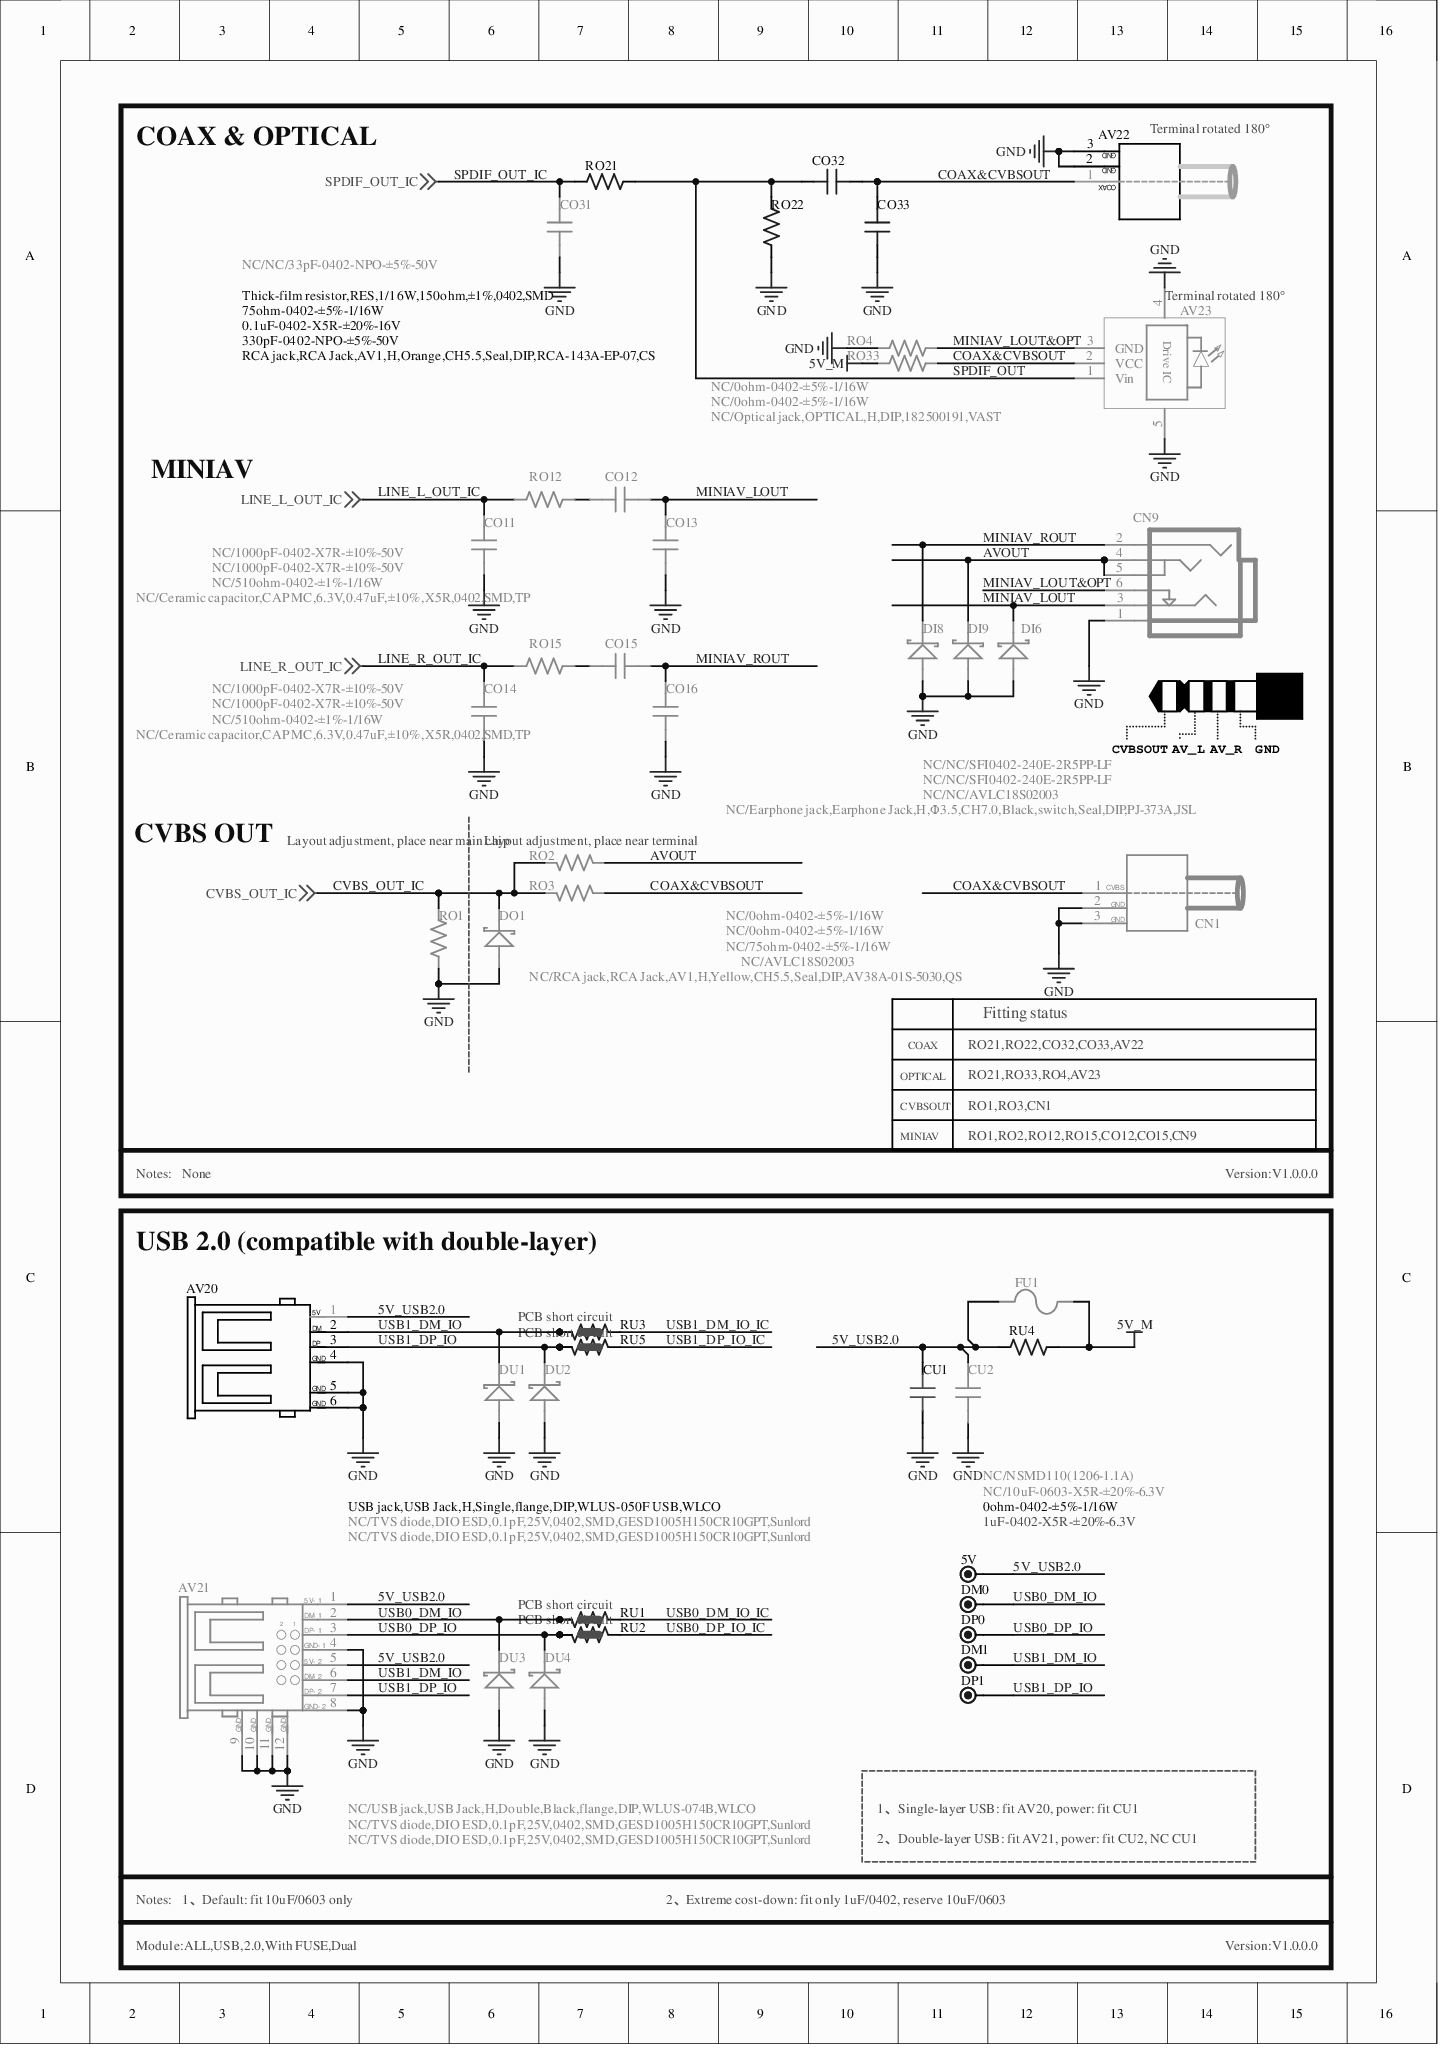
[diagram p0: MISC86372-13.SchDoc]
# Altium project MISC86372-32.PrjPCB (part 5 of 8)

## Sheet MISC86372-13.SchDoc
size 241 x 342 mm

### Parts
5V  DM0  [TP]  (value not drawn)
AV20  USB jack,USB Jack,H,Single,flange,DIP,WLUS-050F USB,WLCO  [USB1-HD-2]
AV21  NC/USB jack,USB Jack,H,Double,Black,flange,DIP,WLUS-074B,WLCO  [USB2-HD-1]
AV22  RCA jack,RCA Jack,AV1,H,Orange,CH5.5,Seal,DIP,RCA-143A-EP-07,CS  [AV1-H-4]
AV23  NC/Optical jack,OPTICAL,H,DIP,182500191,VAST  [OPTICAL-HD-3]
CN1  NC/RCA jack,RCA Jack,AV1,H,Yellow,CH5.5,Seal,DIP,AV38A-01S-5030,QS  [AV1-H-4]
CN9  NC/Earphone jack,Earphone Jack,H,Φ3.5,CH7.0,Black,switch,Seal,DIP,PJ-373A,JSL  [PHONE-HD-42]
CO11  NC/1000pF-0402-X7R-±10%-50V  [C0402]
CO12  NC/Ceramic capacitor,CAP MC,6.3V,0.47uF,±10%,X5R,0402,SMD,TP  [C0402]
CO13  NC/1000pF-0402-X7R-±10%-50V  [C0402]
CO14  NC/1000pF-0402-X7R-±10%-50V  [C0402]
CO15  NC/Ceramic capacitor,CAP MC,6.3V,0.47uF,±10%,X5R,0402,SMD,TP  [C0402]
CO16  NC/1000pF-0402-X7R-±10%-50V  [C0402]
CO31  NC/NC/33pF-0402-NPO-±5%-50V  [C0402]
CO32  0.1uF-0402-X5R-±20%-16V  [C0402]
CO33  330pF-0402-NPO-±5%-50V  [C0402]
CU1  1uF-0402-X5R-±20%-6.3V  [C0402]
CU2  NC/10uF-0603-X5R-±20%-6.3V  [C0603]
DI6  NC/NC/AVLC18S02003  [DIODE-S0402]
DI8  NC/NC/SFI0402-240E-2R5PP-LF  [DIODE-S0402]
DI9  NC/NC/SFI0402-240E-2R5PP-LF  [DIODE-S0402]
DM0  DM0  [TP]  (value not drawn)
DM1  DM0  [TP]  (value not drawn)
DO1  NC/AVLC18S02003  [DIODE-S0402]
DP0  DM0  [TP]  (value not drawn)
DP1  DM0  [TP]  (value not drawn)
DU1  NC/TVS diode,DIO ESD,0.1pF,25V,0402,SMD,GESD1005H150CR10GPT,Sunlord  [DIODE-S0402]
DU2  NC/TVS diode,DIO ESD,0.1pF,25V,0402,SMD,GESD1005H150CR10GPT,Sunlord  [DIODE-S0402]
DU3  NC/TVS diode,DIO ESD,0.1pF,25V,0402,SMD,GESD1005H150CR10GPT,Sunlord  [DIODE-S0402]
DU4  NC/TVS diode,DIO ESD,0.1pF,25V,0402,SMD,GESD1005H150CR10GPT,Sunlord  [DIODE-S0402]
FU1  NC/NSMD110(1206-1.1A)  [FUSE1.1A-S]
RO1  NC/75ohm-0402-±5%-1/16W  [R0402]
RO2  NC/0ohm-0402-±5%-1/16W  [R0402]
RO3  NC/0ohm-0402-±5%-1/16W  [R0402]
RO4  NC/0ohm-0402-±5%-1/16W  [R0402]
RO12  NC/510ohm-0402-±1%-1/16W  [R0402]
RO15  NC/510ohm-0402-±1%-1/16W  [R0402]
RO21  Thick-film resistor,RES,1/16W,150ohm,±1%,0402,SMD  [R0402]
RO22  75ohm-0402-±5%-1/16W  [R0402]
RO33  NC/0ohm-0402-±5%-1/16W  [R0402]
RU1  NC/0ohm-0402-PCB  [R0402SC]  (value not drawn)
RU2  NC/0ohm-0402-PCB  [R0402SC]  (value not drawn)
RU3  NC/0ohm-0402-PCB  [R0402SC]  (value not drawn)
RU4  0ohm-0402-±5%-1/16W  [R0402]
RU5  NC/0ohm-0402-PCB  [R0402SC]  (value not drawn)

### Blocks framed on the sheet
USB 2.0 (compatible with double-layer): 5V AV20 AV21 CU1 CU2 DM0 DM1 DP0 DP1 DU1-DU4 FU1 RU1-RU5

### Nets
5V_M: FU1.2 RO33.1 RU4.2
GND: AV20.4 AV20.5 AV20.6 AV21.4 AV21.8 AV21.9 AV21.10 AV21.11 AV21.12 AV22.2(GND) AV22.3(GND) AV23.4(GND) AV23.5(GND) CN1.2(GND) CN1.3(GND) CN9.1 CO11.1 CO13.1 CO14.1 CO16.1 CO31.1 CO33.1 CU1.2 CU2.2 DI6.A DI8.A DI9.A DO1.A DU1.A DU2.A DU3.A DU4.A RO1.1 RO4.1 RO22.1
5V_USB2.0: 5V.1 AV20.1 AV21.1 AV21.5 CU1.1 CU2.1 FU1.1 RU4.1
AVOUT: CN9.4 CN9.5 DI9.K RO2.1
COAX&CVBSOUT: AV22.1(CVBS) AV23.2(VCC) CN1.1(CVBS) CO32.1 CO33.2 RO3.1 RO33.2
CVBS_OUT_IC: DO1.K RO1.2 RO2.2 RO3.2 ; off-sheet CVBS_OUT_IC
LINE_L_OUT_IC: CO11.2 RO12.2 ; off-sheet LINE_L_OUT_IC
LINE_R_OUT_IC: CO14.2 RO15.2 ; off-sheet LINE_R_OUT_IC
MINIAV_LOUT: CN9.3 CO12.1 CO13.2 DI6.K
MINIAV_LOUT&OPT: AV23.3(GND) CN9.6 RO4.2
MINIAV_ROUT: CN9.2 CO15.1 CO16.2 DI8.K
SPDIF_OUT: AV23.1(Vin) CO32.2 RO21.2 RO22.2
SPDIF_OUT_IC: CO31.2 RO21.1 ; off-sheet SPDIF_OUT_IC
USB0_DM_IO: AV21.2 DM0.1 DU3.K RU1.2 RU1.3
USB0_DM_IO_IC: RU1.1
USB0_DP_IO: AV21.3 DP0.1 DU4.K RU2.2 RU2.3
USB0_DP_IO_IC: RU2.1
USB1_DM_IO: AV20.2 AV21.6 DM1.1 DU1.K RU3.2 RU3.3
USB1_DM_IO_IC: RU3.1
USB1_DP_IO: AV20.3 AV21.7 DP1.1 DU2.K RU5.2 RU5.3
USB1_DP_IO_IC: RU5.1
NetCO12_2: CO12.2 RO12.1
NetCO15_2: CO15.2 RO15.1

### Notes on the sheet
- COAX & OPTICAL
- (near AV22) Terminal rotated 180°
- (near AV23) Terminal rotated 180°
- MINIAV
- CVBSOUT
- AV_L
- AV_R
- GND
- CVBS OUT
- (near RO2) Layout adjustment, place near main chip
- (near RO2) Layout adjustment, place near terminal
- Fitting status
- OPTICAL
- COAX
- RO21,RO22,CO32,CO33,AV22
- RO21,RO33,RO4,AV23
- RO1,RO3,CN1
- RO1,RO2,RO12,RO15,CO12,CO15,CN9
- Notes:
- None
- Version:V1.0.0.0
- 1、 Single-layer USB: fit AV20, power: fit CU1
- 2、 Double-layer USB: fit AV21, power: fit CU2, NC CU1
- 1、 Default: fit 10uF/0603 only
- 2、 Extreme cost-down: fit only 1uF/0402, reserve 10uF/0603
- Module:ALL,USB,2.0,With FUSE,Dual

### Library data of the parts
5V DM0 DM1 DP0 DP1 = TEST
AV20 = XXX.XXX.0002687: USB jack,USB Jack,H,Single,flange,DIP,103411271,VAST-DLMI
AV21 = XXX.XXX.0001070-DLMI: USB jack,USB Jack,H,Double,Black,flange,DIP,WLUS-074B,WLCO-DLMI; Revision: *
AV22 = RCA端子,RCA Jack,AV1,H,Orange,CH5.5,Seal,DIP,AV38A-01S-5020,QS-DLMI
AV23 = 光纤端子,OPTICAL,H,DIP,GQ-03-08C1,QS-DLMI: CN-DLMI-optical fibre
CN1 = RCA端子,RCA Jack,AV1,H,Yellow,CH5.5,Seal,DIP,AV38A-01S-5030,QS-DLMI
CN9 = XXX.XXX.0002138: Earphone jack,Earphone Jack,H,Φ3.5,CH7.0,Black,switch,Seal,DIP,PJ7724-F05L3BY-D,YUQIU-DLMI
CO11 CO13 CO14 CO16 = 1000pF-0402-X7R-±10%-50V-D
CO12 CO15 = 004.003.0000361-D: Ceramic capacitor,CAP MC,6.3V,0.47uF,±10%,X5R,0402,SMD,TP-D
CO31 = 33pF-0402-NPO-±5%-50V-D
CO32 = 004.003.0000403-D: Ceramic capacitor,CAP MC,16V,0.1uF,±20%,X5R,0402,SMD,TP-D
CO33 = 330pF-0402-NPO-±5%-50V-D
CU1 = 1uF-0402-X5R-±20%-6.3V-D
CU2 = 10uF-0603-X5R-±20%-6.3V-D
DI6 DO1 = AVLC18S02003-D
DI8 DI9 = SFI0402-240E-2R5PP-LF-D
DU1-DU4 = 004.005.0000203-D: TVS diode,DIO ESD,0.2pF,25V,0402,SMD,AIES12U020R2,AMOTECH-D
FU1 = 004.026.0000039-D: Self-recovering fuse,FUSE PTC,1.1A,6V,1206,SMD,TP,TLC-D
RO1 = 75ohm-0402-±5%-1/16W-D
RO2 RO3 RU4 = 004.002.0000558-D: Thick-film resistor,RES,1/16W,0ohm,±5%,0402,SMD-D
RO4 RO33 = 0ohm-0402-±5%-1/16W-D
RO12 RO15 = 510ohm-0402-±5%-1/16W-D
RO21 = 004.002.0000609-D: Thick-film resistor,RES,1/16W,180ohm,±5%,0402,SMD-D
RO22 = 004.002.0000568-D: Thick-film resistor,RES,1/16W,100ohm,±5%,0402,SMD-D
RU1-RU3 RU5 = 0ohm-0402-PCB-D

## Sheet MISC86372-14.SchDoc
size 393 x 368 mm
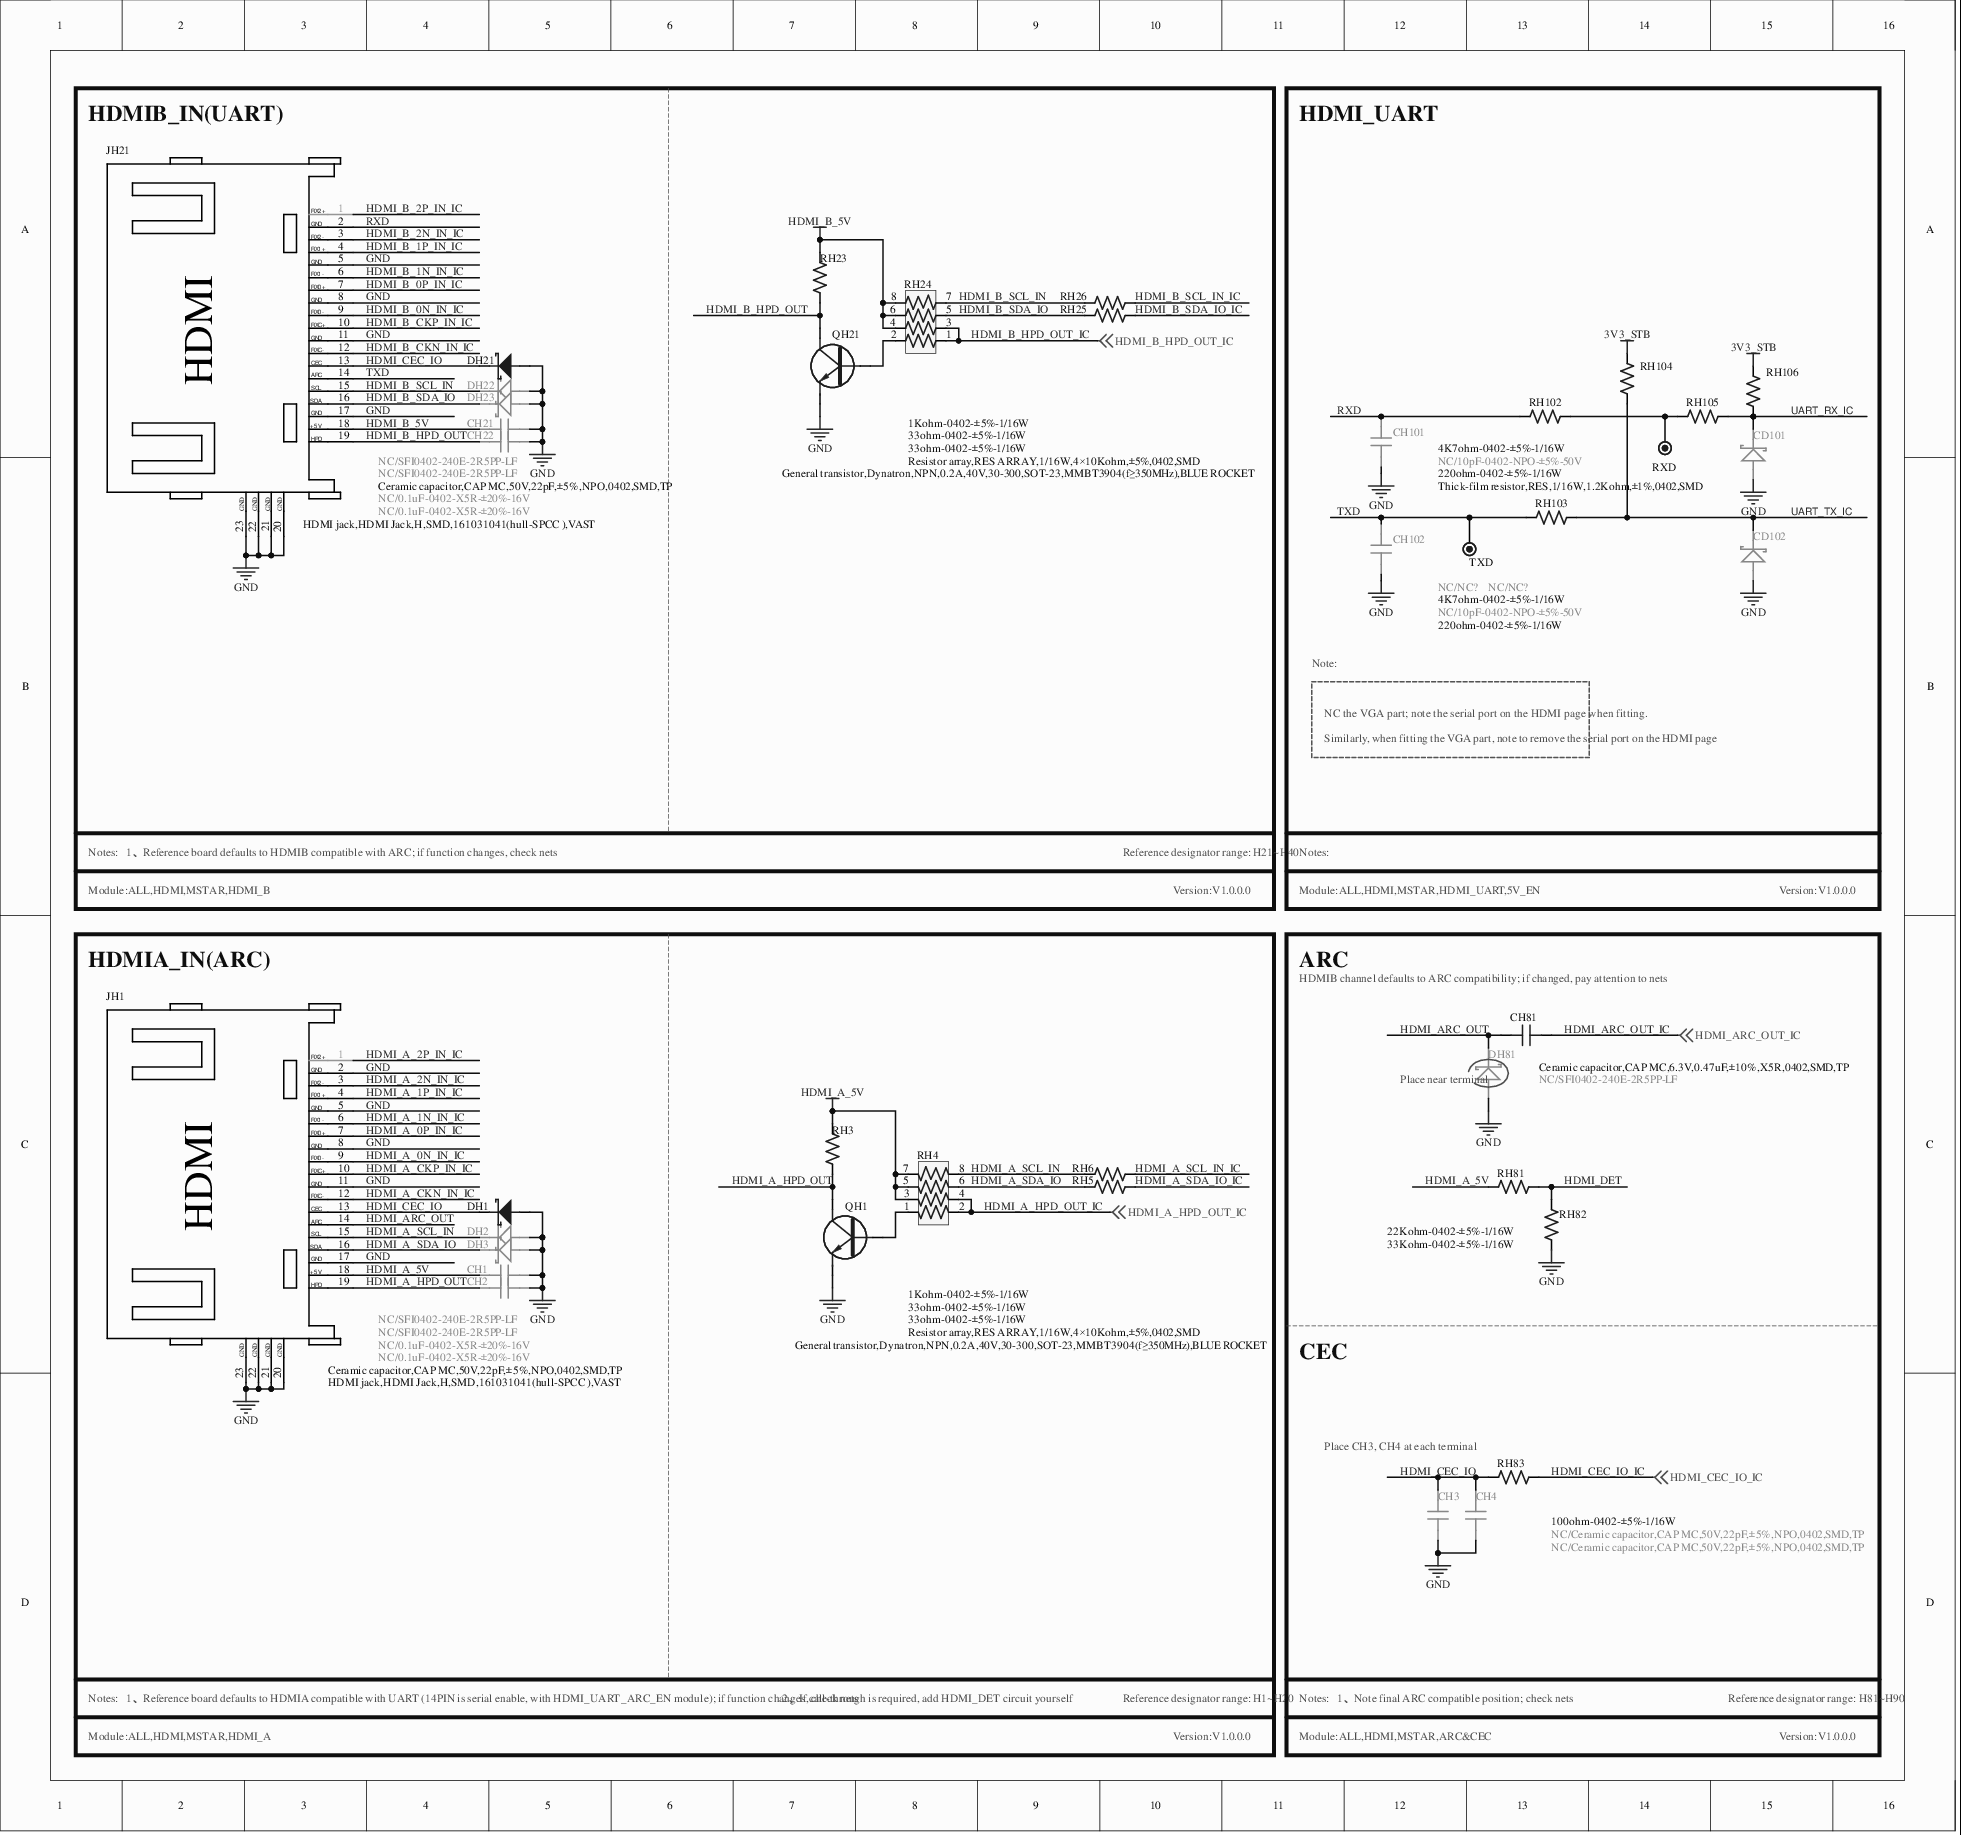
[diagram p1: MISC86372-14.SchDoc]

### Parts
CD101  NC/NC?  [DIODE-S0402]
CD102  NC/NC?  [DIODE-S0402]
CH1  NC/0.1uF-0402-X5R-±20%-16V  [C0402]
CH2  NC/0.1uF-0402-X5R-±20%-16V  [C0402]
CH3  NC/Ceramic capacitor,CAP MC,50V,22pF,±5%,NPO,0402,SMD,TP  [C0402]
CH4  NC/Ceramic capacitor,CAP MC,50V,22pF,±5%,NPO,0402,SMD,TP  [C0402]
CH21  NC/0.1uF-0402-X5R-±20%-16V  [C0402]
CH22  NC/0.1uF-0402-X5R-±20%-16V  [C0402]
CH81  Ceramic capacitor,CAP MC,6.3V,0.47uF,±10%,X5R,0402,SMD,TP  [C0402]
CH101  NC/10pF-0402-NPO-±5%-50V  [C0402]
CH102  NC/10pF-0402-NPO-±5%-50V  [C0402]
DH1  Ceramic capacitor,CAP MC,50V,22pF,±5%,NPO,0402,SMD,TP  [DIODE-S0402]
DH2  NC/SFI0402-240E-2R5PP-LF  [DIODE-S0402]
DH3  NC/SFI0402-240E-2R5PP-LF  [DIODE-S0402]
DH21  Ceramic capacitor,CAP MC,50V,22pF,±5%,NPO,0402,SMD,TP  [DIODE-S0402]
DH22  NC/SFI0402-240E-2R5PP-LF  [DIODE-S0402]
DH23  NC/SFI0402-240E-2R5PP-LF  [DIODE-S0402]
DH81  NC/SFI0402-240E-2R5PP-LF  [DIODE-S0402]
JH1  HDMI jack,HDMI Jack,H,SMD,161031041(hull-SPCC ),VAST  [HDMI-HS-1]
JH21  HDMI jack,HDMI Jack,H,SMD,161031041(hull-SPCC ),VAST  [HDMI-HS-1]
QH1  General transistor,Dynatron,NPN,0.2A,40V,30-300,SOT-23,MMBT3904(f≥350MHz),BLUE ROCKET  [SOT-23]
QH21  General transistor,Dynatron,NPN,0.2A,40V,30-300,SOT-23,MMBT3904(f≥350MHz),BLUE ROCKET  [SOT-23]
RH3  1Kohm-0402-±5%-1/16W  [R0402]
RH4  Resistor array,RES ARRAY,1/16W,4×10Kohm,±5%,0402,SMD  [RA0402]
RH5  33ohm-0402-±5%-1/16W  [R0402]
RH6  33ohm-0402-±5%-1/16W  [R0402]
RH23  1Kohm-0402-±5%-1/16W  [R0402]
RH24  Resistor array,RES ARRAY,1/16W,4×10Kohm,±5%,0402,SMD  [RA0402]
RH25  33ohm-0402-±5%-1/16W  [R0402]
RH26  33ohm-0402-±5%-1/16W  [R0402]
RH81  22Kohm-0402-±5%-1/16W  [R0402]
RH82  33Kohm-0402-±5%-1/16W  [R0402]
RH83  100ohm-0402-±5%-1/16W  [R0402]
RH102  Thick-film resistor,RES,1/16W,1.2Kohm,±1%,0402,SMD  [R0402]
RH103  220ohm-0402-±5%-1/16W  [R0402]
RH104  4K7ohm-0402-±5%-1/16W  [R0402]
RH105  220ohm-0402-±5%-1/16W  [R0402]
RH106  4K7ohm-0402-±5%-1/16W  [R0402]
RXD  (no value)  [TP]
TXD  (no value)  [TP]

### Blocks framed on the sheet
HDMIB_IN(UART): CH21 CH22 DH21-DH23 JH21 QH21 RH23-RH26
HDMI_UART: CD101 CD102 CH101 CH102 RH102-RH106 RXD TXD
HDMIA_IN(ARC): CH1 CH2 DH1-DH3 JH1 QH1 RH3-RH6

### Nets
3V3_STB: RH104.2 RH106.2
GND: CD101.A CD102.A CH1.2 CH2.2 CH3.1 CH4.1 CH21.2 CH22.2 CH101.1 CH102.1 DH1.A DH2.A DH3.A DH21.A DH22.A DH23.A DH81.A JH1.2 JH1.5 JH1.8 JH1.11 JH1.17 JH1.20 JH1.21 JH1.22 JH1.23 JH21.5 JH21.8 JH21.11 JH21.17 JH21.20 JH21.21 JH21.22 JH21.23 QH1.E QH21.E RH82.2
HDMI_A_5V: CH1.1 JH1.18 RH3.2 RH4.3 RH4.5 RH4.7 RH81.2
HDMI_B_5V: CH21.1 JH21.18 RH23.2 RH24.4 RH24.6 RH24.8
HDMI_A_0N_IN_IC: JH1.9
HDMI_A_0P_IN_IC: JH1.7
HDMI_A_1N_IN_IC: JH1.6
HDMI_A_1P_IN_IC: JH1.4
HDMI_A_2N_IN_IC: JH1.3
HDMI_A_2P_IN_IC: JH1.1
HDMI_A_CKN_IN_IC: JH1.12
HDMI_A_CKP_IN_IC: JH1.10
HDMI_A_HPD_OUT: CH2.1 JH1.19 QH1.C RH3.1
HDMI_A_HPD_OUT_IC: RH4.2 RH4.4 ; off-sheet HDMI_A_HPD_OUT_IC
HDMI_A_SCL_IN: DH2.K JH1.15 RH4.8 RH6.1
HDMI_A_SCL_IN_IC: RH6.2
HDMI_A_SDA_IO: DH3.K JH1.16 RH4.6 RH5.1
HDMI_A_SDA_IO_IC: RH5.2
HDMI_ARC_OUT: CH81.1 DH81.K JH1.14
HDMI_ARC_OUT_IC: CH81.2 ; off-sheet HDMI_ARC_OUT_IC
HDMI_B_0N_IN_IC: JH21.9
HDMI_B_0P_IN_IC: JH21.7
HDMI_B_1N_IN_IC: JH21.6
HDMI_B_1P_IN_IC: JH21.4
HDMI_B_2N_IN_IC: JH21.3
HDMI_B_2P_IN_IC: JH21.1
HDMI_B_CKN_IN_IC: JH21.12
HDMI_B_CKP_IN_IC: JH21.10
HDMI_B_HPD_OUT: CH22.1 JH21.19 QH21.C RH23.1
HDMI_B_HPD_OUT_IC: RH24.1 RH24.3 ; off-sheet HDMI_B_HPD_OUT_IC
HDMI_B_SCL_IN: DH22.K JH21.15 RH24.7 RH26.1
HDMI_B_SCL_IN_IC: RH26.2
HDMI_B_SDA_IO: DH23.K JH21.16 RH24.5 RH25.1
HDMI_B_SDA_IO_IC: RH25.2
HDMI_CEC_IO: CH3.2 CH4.2 DH1.K DH21.K JH1.13 JH21.13 RH83.2
HDMI_CEC_IO_IC: RH83.1 ; off-sheet HDMI_CEC_IO_IC
HDMI_DET: RH81.1 RH82.1
RXD: CH101.2 JH21.2 RH102.1
TXD: CH102.2 JH21.14 RH103.1 TXD.1
UART_RX_IC: CD101.K RH105.2 RH106.1
UART_TX_IC: CD102.K RH103.2 RH104.1
NetQH1_B: QH1.B RH4.1
NetQH21_B: QH21.B RH24.2
NetRH102_2: RH102.2 RH105.1 RXD.1

### Notes on the sheet
- Note:
- NC the VGA part; note the serial port on the HDMI page when fitting.
- Similarly, when fitting the VGA part, note to remove the serial port on the HDMI page
- Module:ALL,HDMI,MSTAR,HDMI_B
- Notes:
- 1、 Reference board defaults to HDMIB compatible with ARC; if function changes, check nets
- Reference designator range: H21~H40
- Version:V1.0.0.0
- Module:ALL,HDMI,MSTAR,HDMI_UART,5V_EN
- ARC
- HDMIB channel defaults to ARC compatibility; if changed, pay attention to nets
- (near DH81) Place near terminal
- CEC
- (near RH83) Place CH3, CH4 at each terminal
- 1、 Reference board defaults to HDMIA compatible with UART (14PIN is serial enable, with HDMI_UART_ARC_EN module); if function changes, check nets
- 2、 If call-through is required, add HDMI_DET circuit yourself
- Reference designator range: H1~H20
- 1、 Note final ARC compatible position; check nets
- Reference designator range: H81~H90
- Module:ALL,HDMI,MSTAR,HDMI_A
- Module:ALL,HDMI,MSTAR,ARC&CEC

### Library data of the parts
CD101 CD102 = AVLC18S02003-D
CH1 CH2 CH21 CH22 = 0.1uF-0402-X5R-±20%-16V-D
CH3 CH4 = 004.003.0000530-D: Ceramic capacitor,CAP MC,50V,22pF,±5%,NPO,0402,SMD,TP-D
CH81 = 1uF-0402-X5R-±20%-6.3V-D
CH101 CH102 = 220pF-0402-X7R-±10%-50V-D
DH1-DH3 DH21-DH23 DH81 = 004.005.0000315-D: TVS diode,DIO ESD,2.5pF,200V,0402,SMD,SFI0402-240E-2R5PP-LF,SFI-D
JH1 JH21 = XXX.XXX.0001122-D: HDMI jack,HDMI Jack,H,SMD,161031041(hull-SPCC ),VAST-D
QH1 QH21 = 004.006.0000007-D: General transistor,Dynatron,NPN,0.2A,40V,60-300,SOT-23,KMBT3904,KEXIN-D
RH3 RH23 = 1Kohm-0402-±5%-1/16W-D
RH4 RH24 = 4*100ohm-0402-±5%-1/16W-D
RH5 RH6 RH25 RH26 = 33ohm-0402-±5%-1/16W-D
RH81 = 22Kohm-0402-±5%-1/16W-D
RH82 = 33Kohm-0402-±5%-1/16W-D
RH83 = 004.002.0000568-D: as RO22 on sheet MISC86372-13
RH102-RH106 = 68ohm-0402-±5%-1/16W-D
RXD TXD = TEST

## Sheet MISC86372-15.SchDoc
size 294 x 304 mm
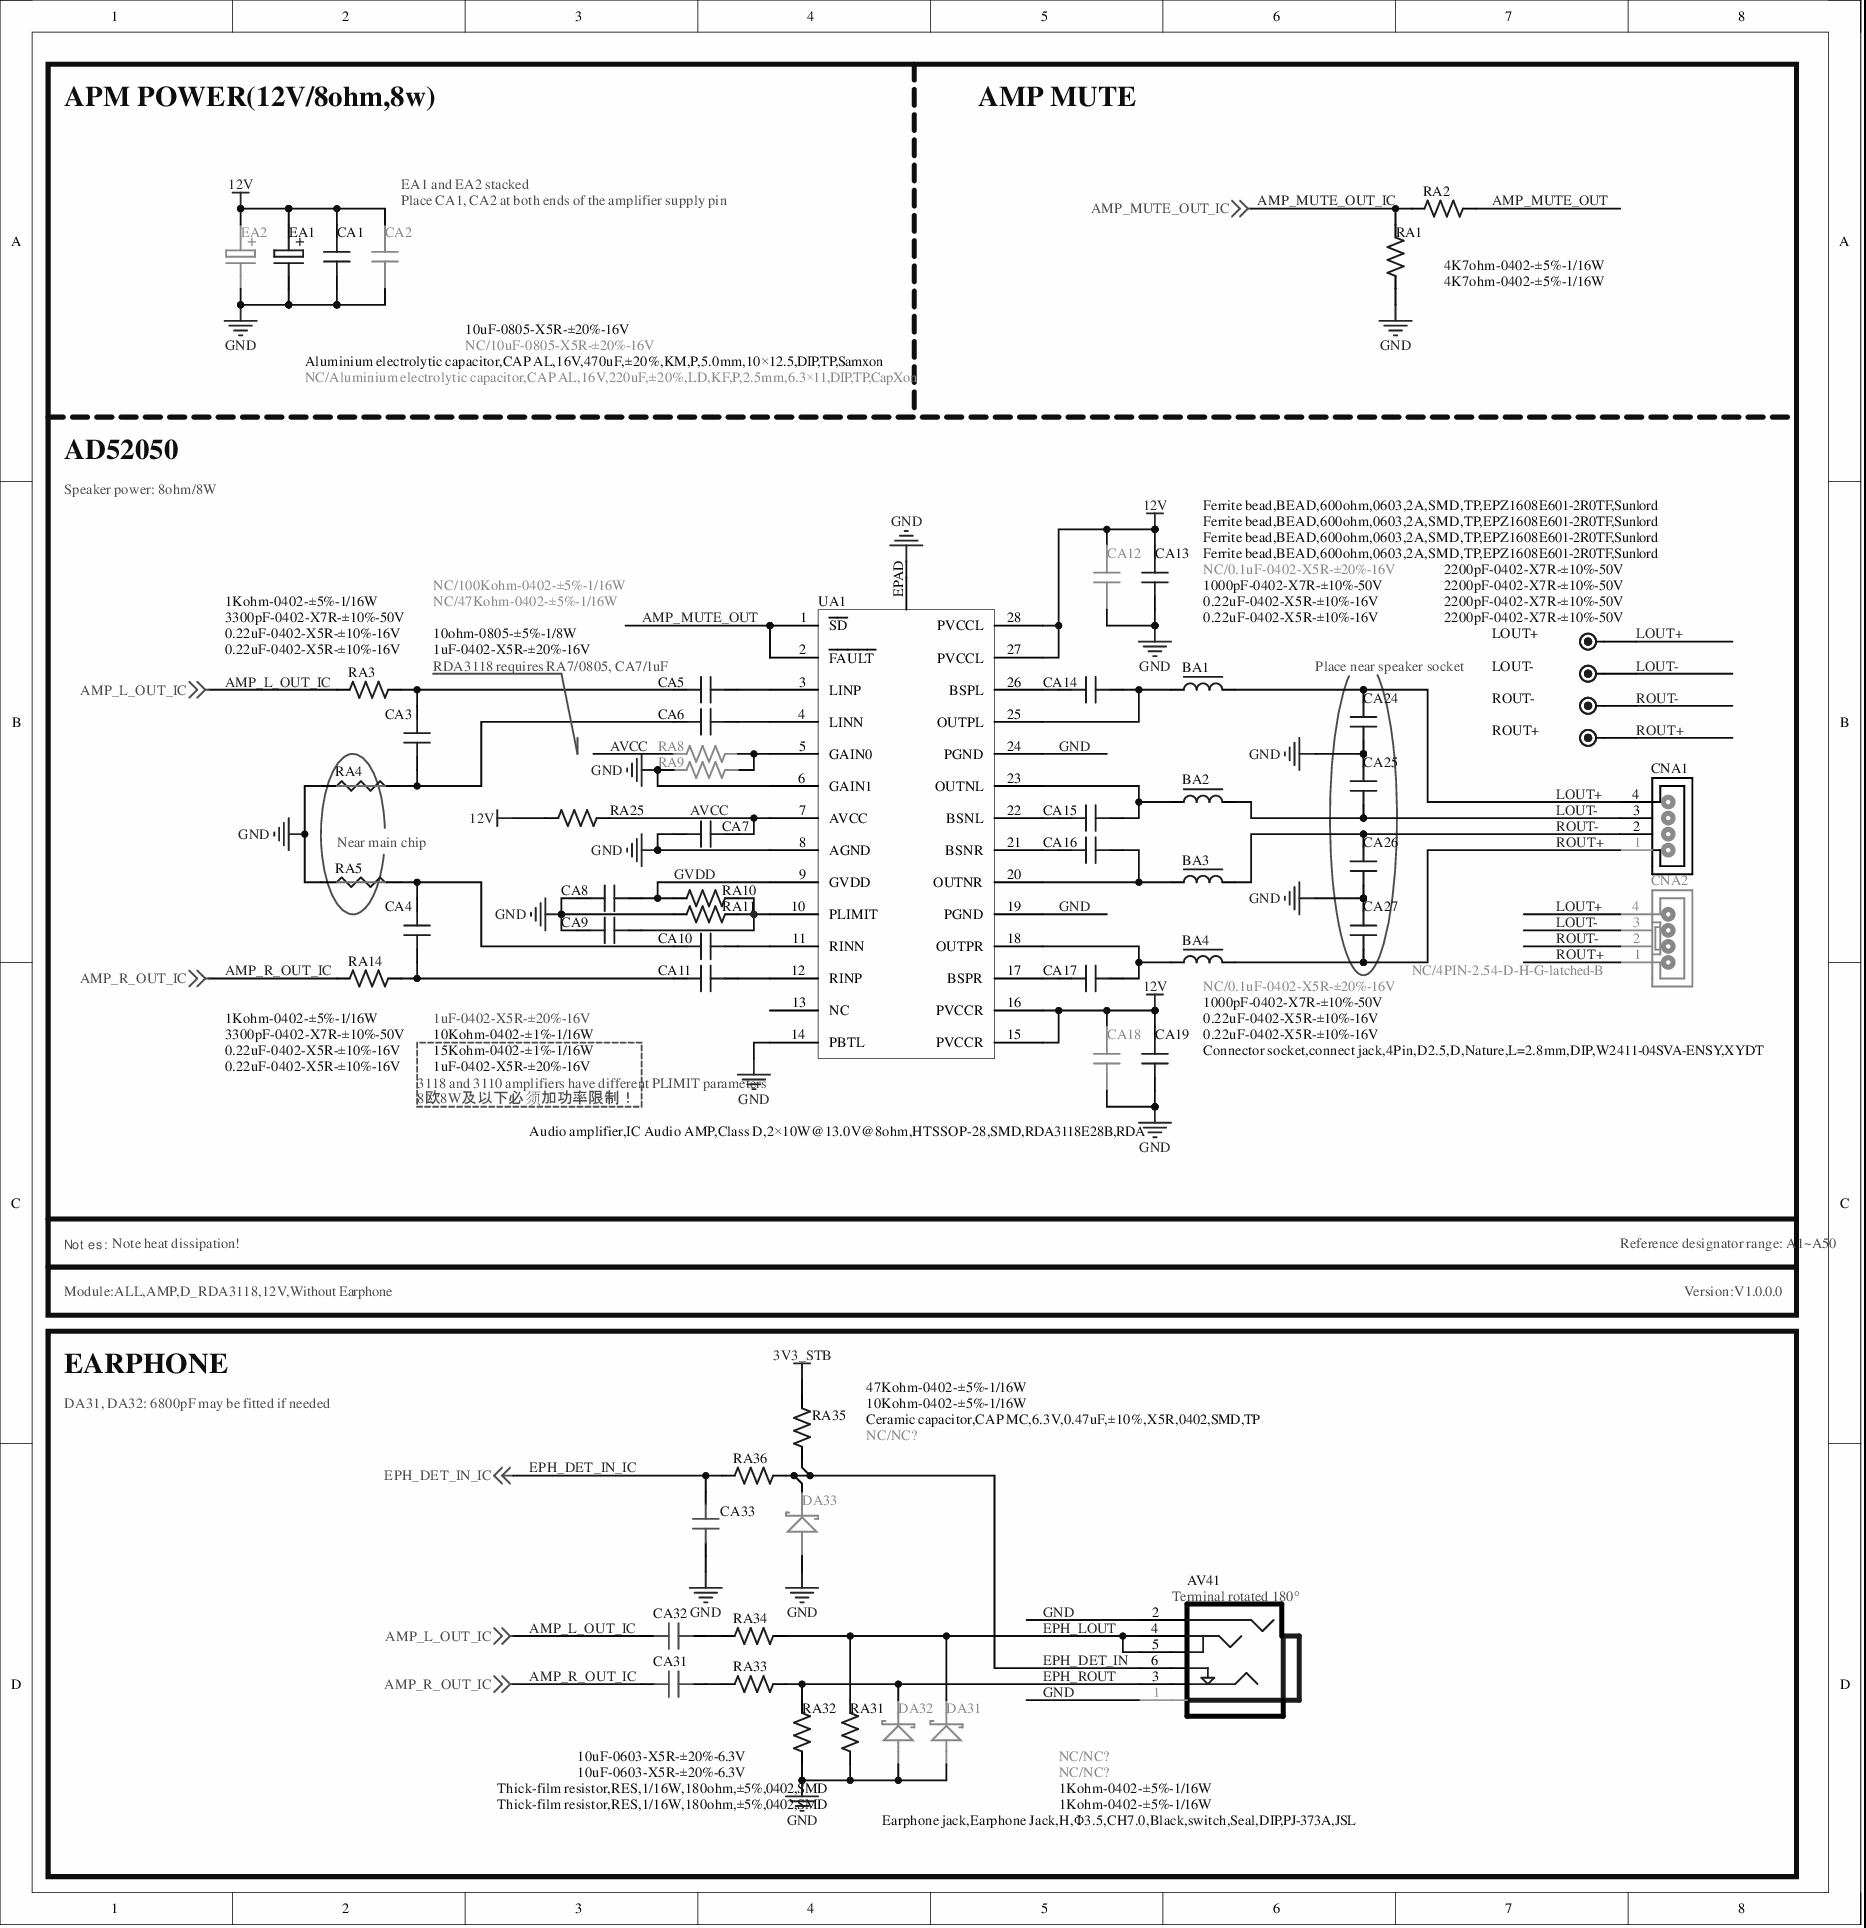
[diagram p2: MISC86372-15.SchDoc]

### Parts
AV41  Earphone jack,Earphone Jack,H,Φ3.5,CH7.0,Black,switch,Seal,DIP,PJ-373A,JSL  [PHONE-HD-42]
BA1  Ferrite bead,BEAD,600ohm,0603,2A,SMD,TP,EPZ1608E601-2R0TF,Sunlord  [L0603]
BA2  Ferrite bead,BEAD,600ohm,0603,2A,SMD,TP,EPZ1608E601-2R0TF,Sunlord  [L0603]
BA3  Ferrite bead,BEAD,600ohm,0603,2A,SMD,TP,EPZ1608E601-2R0TF,Sunlord  [L0603]
BA4  Ferrite bead,BEAD,600ohm,0603,2A,SMD,TP,EPZ1608E601-2R0TF,Sunlord  [L0603]
CA1  10uF-0805-X5R-±20%-16V  [C0805]
CA2  NC/10uF-0805-X5R-±20%-16V  [C0805]
CA3  3300pF-0402-X7R-±10%-50V  [C0402]
CA4  3300pF-0402-X7R-±10%-50V  [C0402]
CA5  0.22uF-0402-X5R-±10%-16V  [C0402]
CA6  0.22uF-0402-X5R-±10%-16V  [C0402]
CA7  1uF-0402-X5R-±20%-16V  [C0402]
CA8  1uF-0402-X5R-±20%-16V  [C0402]
CA9  1uF-0402-X5R-±20%-16V  [C0402]
CA10  0.22uF-0402-X5R-±10%-16V  [C0402]
CA11  0.22uF-0402-X5R-±10%-16V  [C0402]
CA12  NC/0.1uF-0402-X5R-±20%-16V  [C0402]
CA13  1000pF-0402-X7R-±10%-50V  [C0402]
CA14  0.22uF-0402-X5R-±10%-16V  [C0402]
CA15  0.22uF-0402-X5R-±10%-16V  [C0402]
CA16  0.22uF-0402-X5R-±10%-16V  [C0402]
CA17  0.22uF-0402-X5R-±10%-16V  [C0402]
CA18  NC/0.1uF-0402-X5R-±20%-16V  [C0402]
CA19  1000pF-0402-X7R-±10%-50V  [C0402]
CA24  2200pF-0402-X7R-±10%-50V  [C0402]
CA25  2200pF-0402-X7R-±10%-50V  [C0402]
CA26  2200pF-0402-X7R-±10%-50V  [C0402]
CA27  2200pF-0402-X7R-±10%-50V  [C0402]
CA31  10uF-0603-X5R-±20%-6.3V  [C0603]
CA32  10uF-0603-X5R-±20%-6.3V  [C0603]
CA33  Ceramic capacitor,CAP MC,6.3V,0.47uF,±10%,X5R,0402,SMD,TP  [C0402]
CNA1  Connector socket,connect jack,4Pin,D2.5,D,Nature,L=2.8mm,DIP,W2411-04SVA-ENSY,XYDT  [SIP4/2.54D-1]
CNA2  NC/4PIN-2.54-D-H-G-latched-B  [SIP4/2.5D-2]
DA31  NC/NC?  [DIODE-S0402]
DA32  NC/NC?  [DIODE-S0402]
DA33  NC/NC?  [DIODE-S0402]
EA1  Aluminium electrolytic capacitor,CAP AL,16V,470uF,±20%,KM,P,5.0mm,10×12.5,DIP,TP,Samxon  [EC(10*12)-V-5]
EA2  NC/Aluminium electrolytic capacitor,CAP AL,16V,220uF,±20%,LD,KF,P,2.5mm,6.3×11,DIP,TP,CapXon  [EC(6.3*11)-V-2.5]
LOUT+  DM0  [TP]  (value not drawn)
LOUT-  DM0  [TP]  (value not drawn)
RA1  4K7ohm-0402-±5%-1/16W  [R0402]
RA2  4K7ohm-0402-±5%-1/16W  [R0402]
RA3  1Kohm-0402-±5%-1/16W  [R0402]
RA4  NC/?  [GND]  (value not drawn)
RA5  NC/?  [GND]  (value not drawn)
RA8  NC/100Kohm-0402-±5%-1/16W  [R0402]
RA9  NC/47Kohm-0402-±5%-1/16W  [R0402]
RA10  10Kohm-0402-±1%-1/16W  [R0402]
RA11  15Kohm-0402-±1%-1/16W  [R0402]
RA14  1Kohm-0402-±5%-1/16W  [R0402]
RA25  10ohm-0805-±5%-1/8W  [R0805]
RA31  1Kohm-0402-±5%-1/16W  [R0402]
RA32  1Kohm-0402-±5%-1/16W  [R0402]
RA33  Thick-film resistor,RES,1/16W,180ohm,±5%,0402,SMD  [R0402]
RA34  Thick-film resistor,RES,1/16W,180ohm,±5%,0402,SMD  [R0402]
RA35  47Kohm-0402-±5%-1/16W  [R0402]
RA36  10Kohm-0402-±5%-1/16W  [R0402]
ROUT+  DM0  [TP]  (value not drawn)
ROUT-  DM0  [TP]  (value not drawn)
UA1  Audio amplifier,IC Audio AMP,Class D,2×10W@13.0V@8ohm,HTSSOP-28,SMD,RDA3118E28B,RDA  [SSOP28/0.65-5]

### Blocks framed on the sheet
EARPHONE: AV41 CA31-CA33 DA31-DA33 RA31-RA36

### Nets
3V3_STB: RA35.2
12V: CA1.2 CA2.2 CA12.2 CA13.2 CA18.2 CA19.2 EA1.1 EA2.1 RA25.1 UA1.15(PVCCR) UA1.16(PVCCR) UA1.27(PVCCL) UA1.28(PVCCL)
GND: AV41.1 AV41.2 CA1.1 CA2.1 CA7.1 CA8.1 CA9.1 CA12.1 CA13.1 CA18.1 CA19.1 CA24.1 CA25.2 CA26.1 CA27.2 CA33.1 DA31.A DA32.A DA33.A EA1.2 EA2.2 RA1.2 RA4.JP_2K RA5.JP_2K RA9.1 RA11.1 RA31.1 RA32.1 UA1.6(GAIN1) UA1.8(AGND) UA1.14(PBTL) UA1.19(PGND) UA1.24(PGND) UA1.EPAD
AMP_L_OUT_IC: CA32.2 RA3.1 ; off-sheet AMP_L_OUT_IC
AMP_MUTE_OUT: RA2.1 UA1.1(~{SD}) UA1.2(~{FAULT})
AMP_MUTE_OUT_IC: RA1.1 RA2.2 ; off-sheet AMP_MUTE_OUT_IC
AMP_R_OUT_IC: CA31.2 RA14.1 ; off-sheet AMP_R_OUT_IC
AVCC: CA7.2 RA8.1 RA25.2 UA1.7(AVCC)
EPH_DET_IN: AV41.6 DA33.K RA35.1 RA36.2
EPH_DET_IN_IC: CA33.2 RA36.1 ; off-sheet EPH_DET_IN_IC
EPH_LOUT: AV41.4 AV41.5 DA31.K RA31.2 RA34.2
EPH_ROUT: AV41.3 DA32.K RA32.2 RA33.2
GVDD: CA8.2 RA10.1 UA1.9(GVDD)
LOUT+: BA1.2 CA24.2 CNA1.4 CNA2.4 LOUT+.1
LOUT-: BA2.2 CA25.1 CNA1.3 CNA2.3 LOUT-.1
ROUT+: BA4.2 CA27.1 CNA1.1 CNA2.1 ROUT+.1
ROUT-: BA3.2 CA26.2 CNA1.2 CNA2.2 ROUT-.1
NetBA1_1: BA1.1 CA14.2 UA1.25(OUTPL)
NetBA2_1: BA2.1 CA15.2 UA1.23(OUTNL)
NetBA3_1: BA3.1 CA16.2 UA1.20(OUTNR)
NetBA4_1: BA4.1 CA17.2 UA1.18(OUTPR)
NetCA3_1: CA3.1 CA6.1 RA4.JP_1K
NetCA3_2: CA3.2 CA5.1 RA3.2
NetCA4_1: CA4.1 CA11.1 RA14.2
NetCA4_2: CA4.2 CA10.1 RA5.JP_1K
NetCA5_2: CA5.2 UA1.3(LINP)
NetCA6_2: CA6.2 UA1.4(LINN)
NetCA9_2: CA9.2 RA10.2 RA11.2 UA1.10(PLIMIT)
NetCA10_2: CA10.2 UA1.11(RINN)
NetCA11_2: CA11.2 UA1.12(RINP)
NetCA14_1: CA14.1 UA1.26(BSPL)
NetCA15_1: CA15.1 UA1.22(BSNL)
NetCA16_1: CA16.1 UA1.21(BSNR)
NetCA17_1: CA17.1 UA1.17(BSPR)
NetCA31_1: CA31.1 RA33.1
NetCA32_1: CA32.1 RA34.1
NetRA8_2: RA8.2 RA9.2 UA1.5(GAIN0)

Not connected (* = marked no-connect by the designer): UA1 13(NC)*

### Notes on the sheet
- APM POWER(12V/8ohm,8w)
- AMP MUTE
- (near CA2) EA1 and EA2 stacked
- (near CA2) Place CA1, CA2 at both ends of the amplifier supply pin
- AD52050
- Speaker power: 8ohm/8W
- (near CA5) RDA3118 requires RA7/0805, CA7/1uF
- (near CA24) Place near speaker socket
- Near main chip
- (near UA1) 3118 and 3110 amplifiers have different PLIMIT parameters
- 8欧8W及以下必须加功率限制！
- Notes:
- Module:ALL,AMP,D_RDA3118,12V,Without Earphone
- Note heat dissipation!
- Reference designator range: A1~A50
- Version:V1.0.0.0
- DA31, DA32: 6800pF may be fitted if needed
- (near AV41) Terminal rotated 180°

### Library data of the parts
AV41 = XXX.XXX.0002138: as CN9 on sheet MISC86372-13
BA1-BA4 = 004.004.0000104-D: Multilayer inductor,HF Inductor,220nH,±5%,0603,SMD,SWI0603F-R22J,Tai-tech-D
CA1 CA2 = 004.003.0000386-D: Ceramic capacitor,CAP MC,16V,10uF,±20%,X5R,0805,SMD,TP-D
CA3 CA4 = 004.003.0000549-D: Ceramic capacitor,CAP MC,50V,3300pF,±10%,X7R,0402,SMD,TP-D
CA5 CA6 CA10 CA11 CA14-CA17 = 004.003.0000398-D: Ceramic capacitor,CAP MC,16V,0.22uF,±20%,X5R,0402,SMD,TP-D
CA7 CA9 = 004.003.0000402-D: Ceramic capacitor,CAP MC,16V,1uF,±20%,X5R,0402,SMD,TP-D
CA8 CA12 CA18 = 004.003.0000403-D: as CO32 on sheet MISC86372-13
CA13 CA19 = 004.003.0000503-D: Ceramic capacitor,CAP MC,50V,1000pF,±10%,X7R,0402,SMD,TP-D
CA24-CA27 = 004.003.0000534-D: Ceramic capacitor,CAP MC,50V,2200pF,±10%,X7R,0402,SMD,TP-D
CA31 CA32 = 004.003.0000383-D: Ceramic capacitor,CAP MC,6.3V,10uF,±20%,X5R,0603,SMD,TP-D
CA33 = 004.003.0000361-D: as CO12 on sheet MISC86372-13
CNA1 = XXX.XXX.0000595-DHMI: Connector socket,connect jack,4Pin,D2.50,D,L=2.8mm,DIP,CNJST-DHMI
CNA2 = XXX.XXX.0000676-DHMI: Connector socket,connect jack,4Pin,D2.54,D,SNAP,L=3.0mm,DIP,BOOM-DHMI
DA31-DA33 = AVLC18S02003-D
EA1 = 004.003.0000601-DHAI: Aluminium electrolytic capacitor,CAP AL,16V,470uF,±20%,RK,P,5.0mm,10×12,DIP,TP,XL-DHAI
EA2 = 004.003.0000158-DHAI: Aluminium electrolytic capacitor,CAP AL,16V,220uF,±20%,LD,KF,P,2.5mm,6.3×11,DIP,TP,CapXon-DHAI
LOUT+ LOUT- ROUT+ ROUT- = TEST
RA1 RA2 = 004.002.0000689-D: Thick-film resistor,RES,1/16W,4.7Kohm,±5%,0402,SMD-D
RA3 RA14 = 004.002.0000572-D: Thick-film resistor,RES,1/16W,1Kohm,±5%,0402,SMD-D
RA4 RA5 = GND: Manufacturer: Panasonic; Part Number: ERJ3GEYJ473V; Right: 20; Bottom: 30; CLASS: Discrete; Comments: Digikey
RA8 = 004.002.0000579-D: Thick-film resistor,RES,1/16W,100Kohm,±5%,0402,SMD-D
RA9 = 004.002.0000691-D: Thick-film resistor,RES,1/16W,47Kohm,±5%,0402,SMD-D
RA10 = 004.002.0000575-D: Thick-film resistor,RES,1/16W,10Kohm,±1%,0402,SMD-D
RA11 = 004.002.0000602-D: Thick-film resistor,RES,1/16W,15Kohm,±1%,0402,SMD-D
RA25 = 004.002.0000562-D: Thick-film resistor,RES,1/8W,10ohm,±5%,0805,SMD-D
RA31 RA32 = 1Kohm-0402-±5%-1/16W-D
RA33 RA34 = 004.002.0000609-D: as RO21 on sheet MISC86372-13
RA35 = 47Kohm-0402-±5%-1/16W-D
RA36 = 10Kohm-0402-±5%-1/16W-D
UA1 = 004.012.0000190-D: Audio amplifier,IC Audio AMP,Class D,2×10W@13.0V@8ohm,HTSSOP-28,SMD,RDA3118E28B,RDA-D